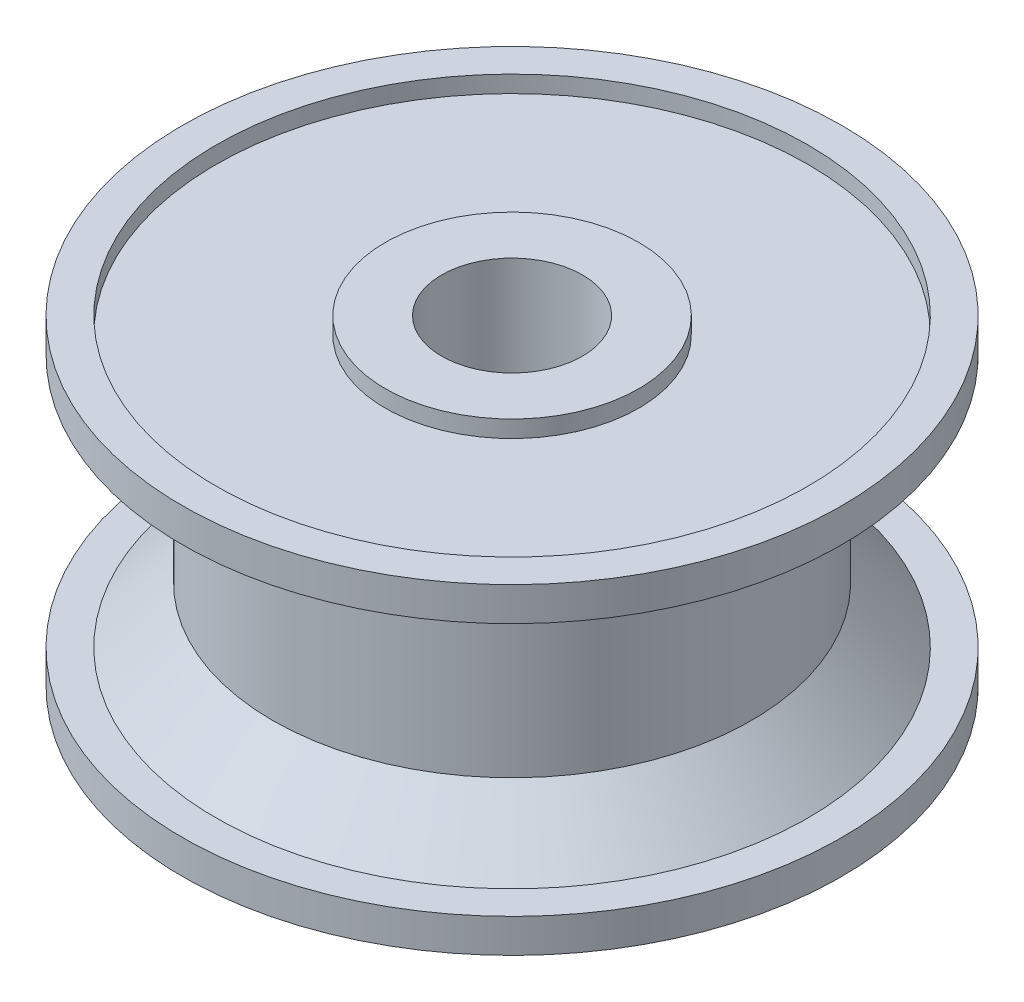
SolidWorks part; units mm, degrees
ref_plane "前视基准面" through (0, 0, 0) normal (0, 0, 1) x (1, 0, 0)
ref_plane "上视基准面" through (0, 0, 0) normal (0, 1, 0) x (1, 0, 0)
ref_plane "右视基准面" through (0, 0, 0) normal (1, 0, 0) x (0, 0, -1)
sketch "草图1" plane through (0, 0, 0) normal (0, 0, 1) x (1, 0, 0)
  line L0 (52.5, 22.5) -> (58.5, 22.5)
  line L1 (52.5, 22.5) -> (42.5, 12.5)
  line L2 (58.5, 28.5) -> (58.5, 22.5)
  line L3 (0, -28.5) -> (58.5, -28.5)
  line L4 (58.5, -28.5) -> (58.5, -22.5)
  line L5 (42.5, 12.5) -> (42.5, -12.5)
  line L6 (52.5, -22.5) -> (42.5, -12.5)
  line L7 (0, 28.5) -> (58.5, 28.5)
  line L8 (0, -28.5) -> (0, 28.5) construction
  line L9 (0, 0) -> (42.5, 0) construction
  line L10 (52.5, -22.5) -> (58.5, -22.5)
  line L11 (0, -28.5) -> (0, 28.5)
  dimension "D1" = 58.5
  dimension "D2" = 28.5
  dimension "D3" = 22.5
  dimension "D4" = 42.5
  dimension "D5" = 135
  dimension "D6" = 12.5
revolve "旋转1" add sketch "草图1" angle 360 about L11
sketch "草图2" plane through (0, -28.5, 0) normal (0, -1, 0) x (1, 0, 0)
  circle A0 centre (0, 0) radius 12.5
  dimension "D1" = 25
extrude "切除-拉伸1" cut sketch "草图2" against normal through all
sketch "草图3" plane through (0, -28.5, 0) normal (0, -1, 0) x (1, 0, 0)
  circle A0 centre (0, 0) radius 52.5
  circle A1 centre (0, 0) radius 22.5
  dimension "D1" = 45
  dimension "D2" = 105
extrude "切除-拉伸2" cut sketch "草图3" against normal blind 3
mirror "镜向1" about plane through (0, 0, 0) normal (0, 1, 0) of "切除-拉伸2"
